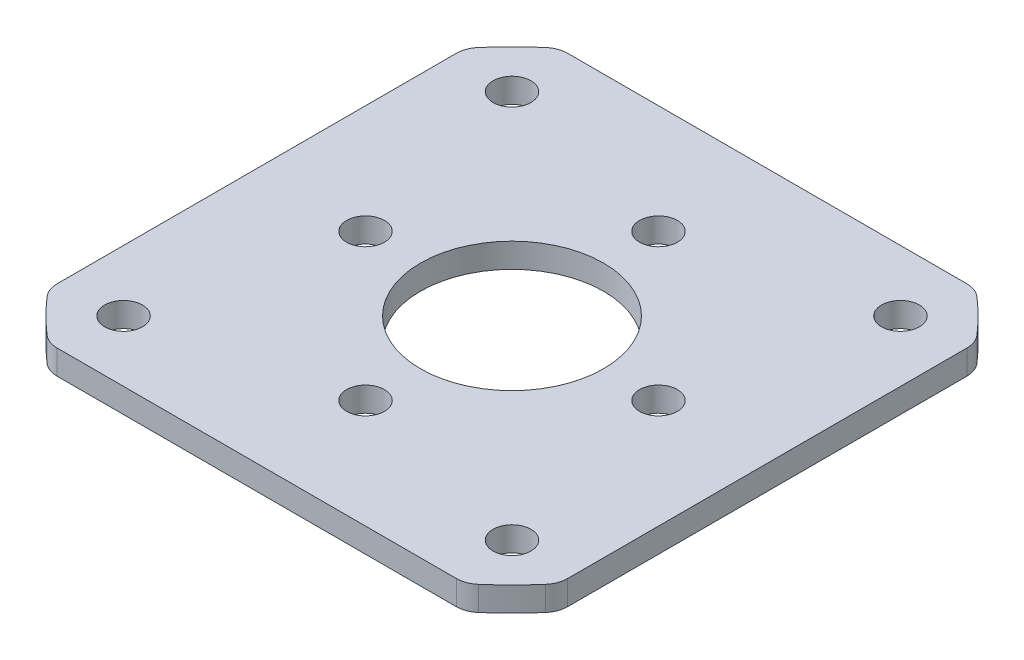
from build123d import *

# Parameters (mm, degrees)
SKETCH_1_R      = 7.5
SKETCH_1_R_2    = 1.55
EXTRUDE_1_DEPTH = 2
FILLET_1_R      = 2


with BuildPart() as part:
    # 草图1 → 凸台-拉伸1 (new body)
    with BuildSketch(Plane(origin=(0, 0, 0), x_dir=(1, 0, 0), z_dir=(0, 1, 0))):
        with BuildLine():
            Line((17.081451175, -20.909902577), (-17.081451175, -20.909902577))
            ThreePointArc((-17.081451175, -20.909902577), (-19.091883092, -19.091883092), (-20.909902577, -17.081451175))
            Line((-20.909902577, -17.081451175), (-20.909902577, 17.081451175))
            ThreePointArc((-20.909902577, 17.081451175), (-19.091883092, 19.091883092), (-17.081451175, 20.909902577))
            Line((-17.081451175, 20.909902577), (17.081451175, 20.909902577))
            ThreePointArc((17.081451175, 20.909902577), (19.091883092, 19.091883092), (20.909902577, 17.081451175))
            Line((20.909902577, 17.081451175), (20.909902577, -17.081451175))
            ThreePointArc((20.909902577, -17.081451175), (19.091883092, -19.091883092), (17.081451175, -20.909902577))
        make_face()
        with Locations(Location((0, 0, 0), (0, 0, 270))):
            Circle(SKETCH_1_R, mode=Mode.SUBTRACT)
        with Locations(Location((12, 0, 0), (0, 0, 270))):
            Circle(SKETCH_1_R_2, mode=Mode.SUBTRACT)
        with Locations(Location((15.909902577, 15.909902577, 0), (0, 0, 270))):
            Circle(SKETCH_1_R_2, mode=Mode.SUBTRACT)
        with Locations(Location((0, -12, 0), (0, 0, 270))):
            Circle(SKETCH_1_R_2, mode=Mode.SUBTRACT)
        with Locations(Location((15.909902577, -15.909902577, 0), (0, 0, 270))):
            Circle(SKETCH_1_R_2, mode=Mode.SUBTRACT)
        with Locations(Location((-12, 0, 0), (0, 0, 270))):
            Circle(SKETCH_1_R_2, mode=Mode.SUBTRACT)
        with Locations(Location((-15.909902577, -15.909902577, 0), (0, 0, 270))):
            Circle(SKETCH_1_R_2, mode=Mode.SUBTRACT)
        with Locations(Location((0, 12, 0), (0, 0, 270))):
            Circle(SKETCH_1_R_2, mode=Mode.SUBTRACT)
        with Locations(Location((-15.909902577, 15.909902577, 0), (0, 0, 270))):
            Circle(SKETCH_1_R_2, mode=Mode.SUBTRACT)
    extrude(amount=EXTRUDE_1_DEPTH)

    # 圆角1
    fillet_1_edges = [part.edges().sort_by_distance(p)[0] for p in [
        (17.081451175, 1, 20.909902577),
        (-17.081451175, 1, 20.909902577),
        (-20.909902577, 1, 17.081451175),
        (-20.909902577, 1, -17.081451175),
        (-17.081451175, 1, -20.909902577),
        (17.081451175, 1, -20.909902577),
        (20.909902577, 1, -17.081451175),
        (20.909902577, 1, 17.081451175),
    ]]
    fillet(fillet_1_edges, radius=FILLET_1_R)


solid = part.part
